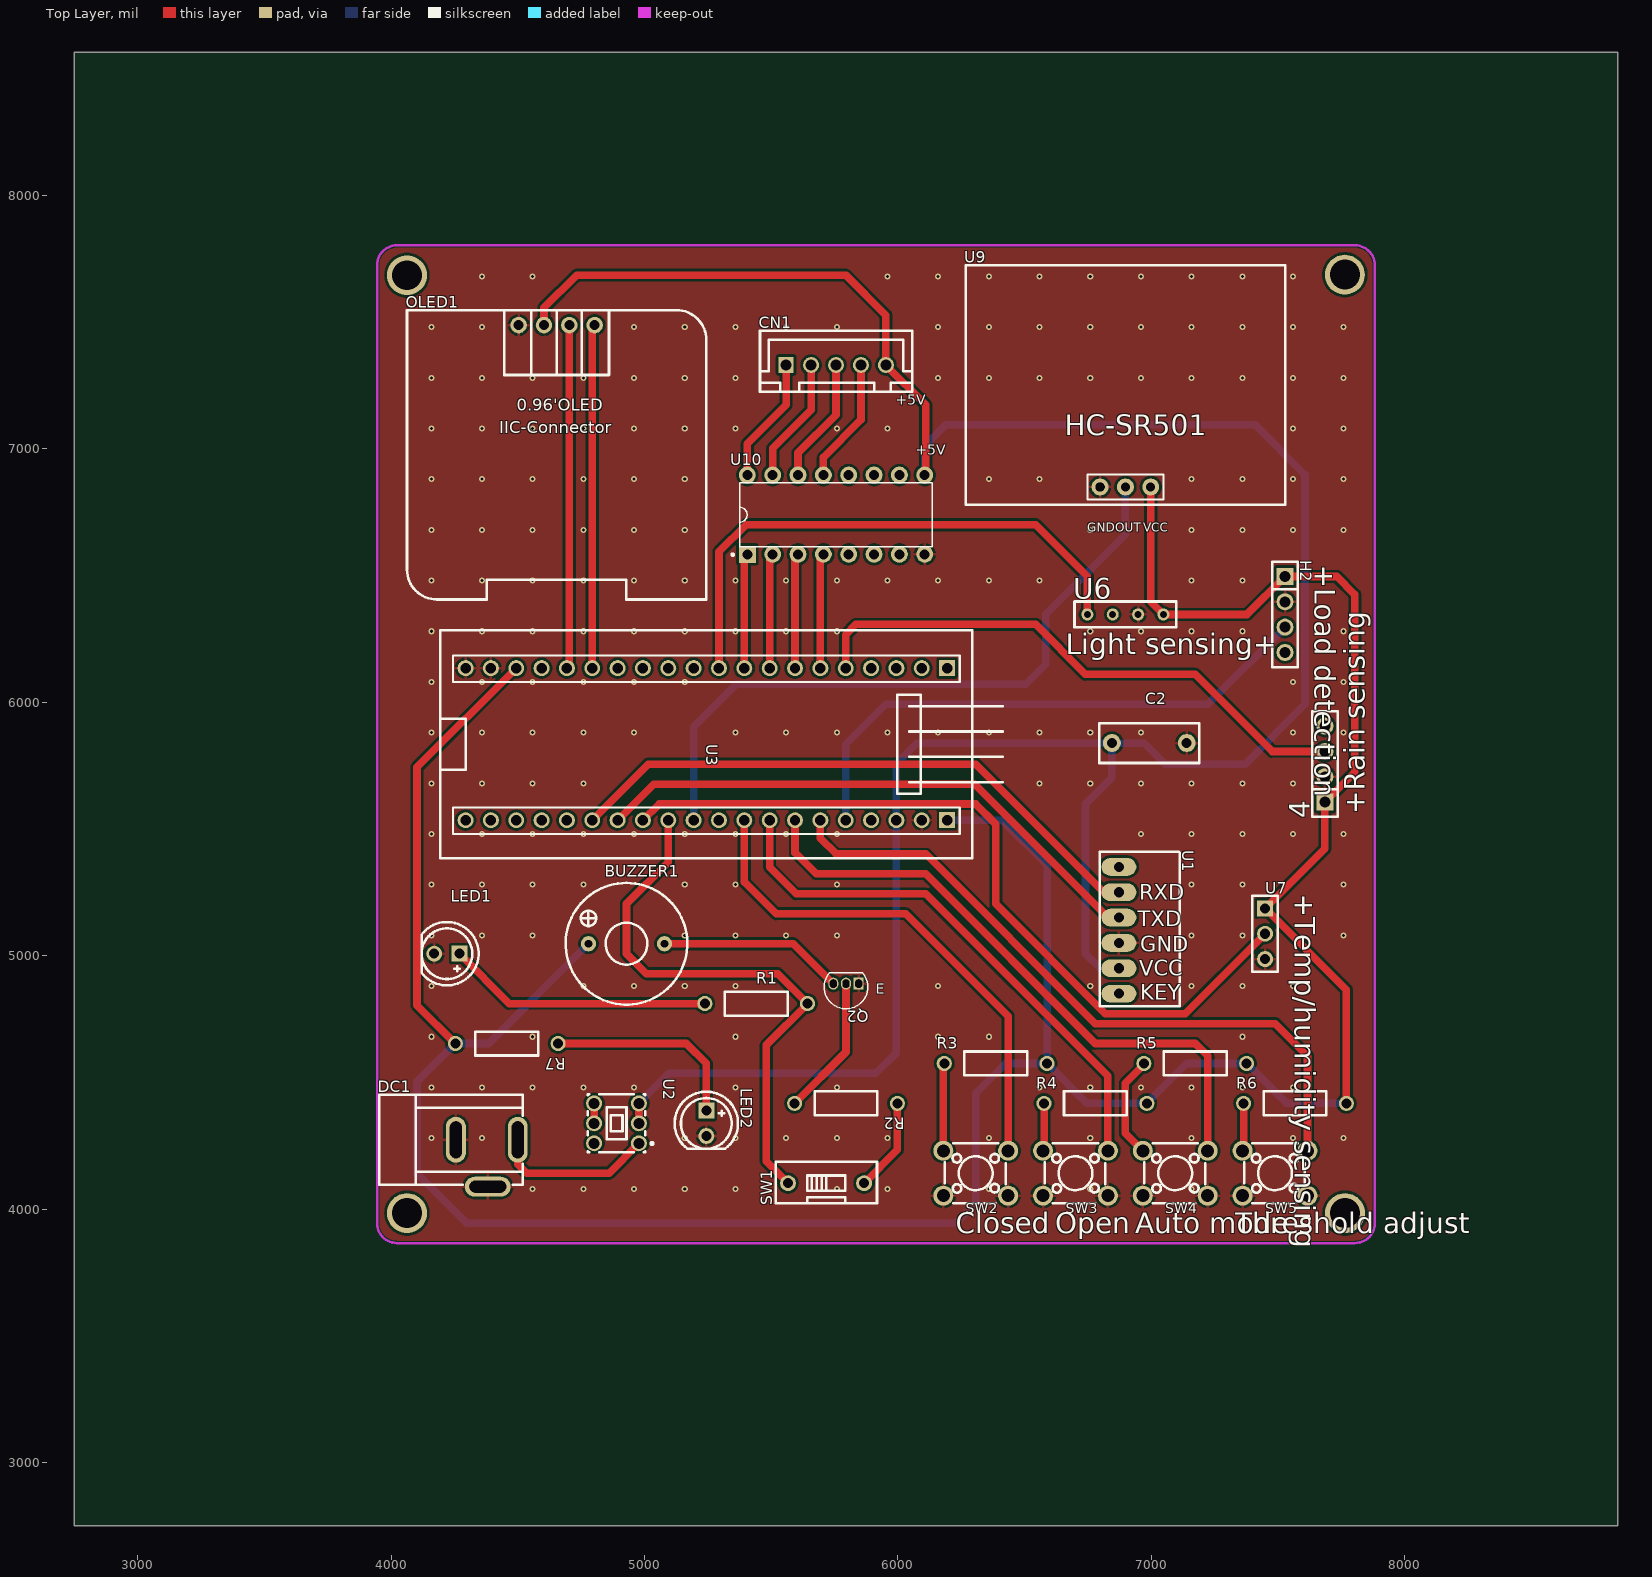
[diagram p0: Top Layer view]
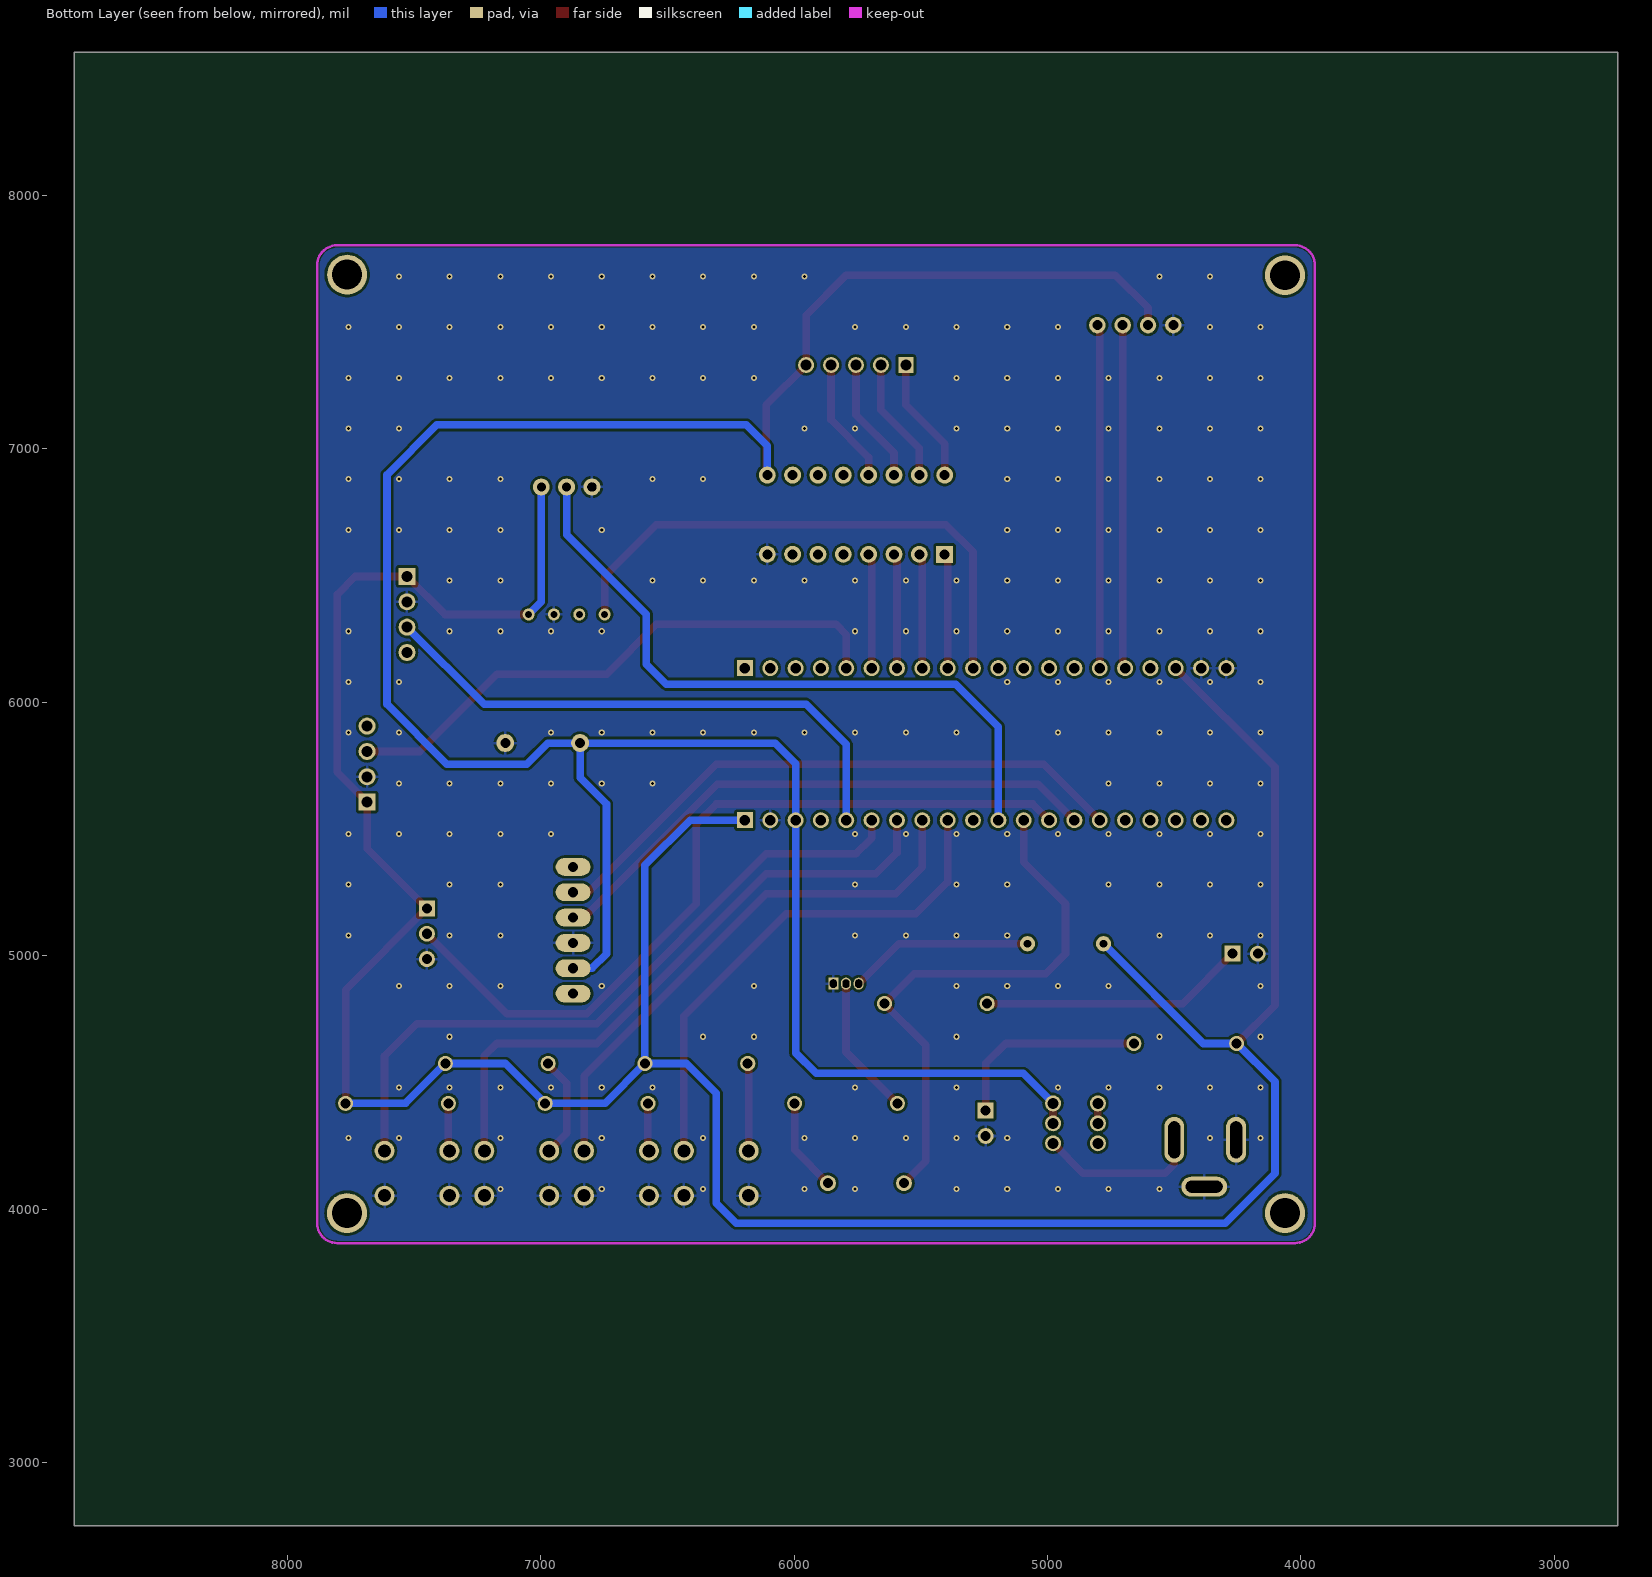
[diagram p1: Bottom Layer view, seen from below]
# Altium PCB MISC61241.pcbdoc
Units mil, origin at the board's own origin, x right, y up, seen from the top; angles counter-clockwise.
Board outline 6090.55 x 5814.96 mil, 2 copper layers (Top Layer, Bottom Layer), stack 62.206 mil thick; 29 components, 36 nets, 145 pads, 225 vias.

## Layer stack, top to bottom
Top Solder Mask Layer: solder mask 0.394, Dk 3.3
Top Layer: signal copper 1.379
Dielectric1: surface 59.449, FR4, Dk 4.5
Bottom Layer: signal copper 1.378
Bottom Solder Mask Layer: solder mask 0.394, Dk 3.3

## Board outline
8840.55,2750 2750,2750 2750,8564.96 8840.55,8564.96

## Design rules (kind name [scope] priority, off if disabled: settings)
BoardOutlineClearance copperThickness2oz_1 [All] p2 off: genericclearance=7.99 ignorepadtopadclearanceinfootprint=FALSE except(0: Arc-SplitContinuation Track-SplitContinuation SMDPad-SplitContinuation THPad-SplitContinuation Via-SplitContinuation Fill-SplitContinuation Region-SplitContinuation Poly-SplitContinuation Text-SplitContinuation Hole-SplitContinuation; 5.98: Arc-CutoutEdge SMDPad-CutoutEdge THPad-CutoutEdge Via-CutoutEdge Fill-CutoutEdge Region-CutoutEdge Text-CutoutEdge; 6.93: Hole-OutlineEdge Hole-CutoutEdge; 10: Poly-OutlineEdge Poly-CutoutEdge; 11.81: Arc-OutlineEdge Track-OutlineEdge SMDPad-OutlineEdge THPad-OutlineEdge Via-OutlineEdge Fill-OutlineEdge Region-OutlineEdge Text-OutlineEdge Track-CutoutEdge)
BoardOutlineClearance copperThickness1oz_1 [All] p4: genericclearance=4.02 ignorepadtopadclearanceinfootprint=FALSE except(0: Arc-SplitContinuation Track-SplitContinuation SMDPad-SplitContinuation THPad-SplitContinuation Via-SplitContinuation Fill-SplitContinuation Region-SplitContinuation Poly-SplitContinuation Text-SplitContinuation Hole-SplitContinuation; 6: SMDPad-CutoutEdge THPad-CutoutEdge Via-CutoutEdge Fill-CutoutEdge Region-CutoutEdge Text-CutoutEdge; 6.93: Hole-OutlineEdge Hole-CutoutEdge; 10: Poly-OutlineEdge Poly-CutoutEdge; 11.8: Arc-OutlineEdge Track-OutlineEdge SMDPad-OutlineEdge THPad-OutlineEdge Via-OutlineEdge Fill-OutlineEdge Region-OutlineEdge Text-OutlineEdge; 11.81: Arc-CutoutEdge Track-CutoutEdge)
Clearance copperThickness2oz [All] p1 off: gap=7.99 ignorepadtopadclearanceinfootprint=FALSE except(5.98: SMDPad-Track SMDPad-SMDPad THPad-Track SMDPad-THPad THPad-THPad Track-Via SMDPad-Via THPad-Via Via-Via Fill-Track Region-Track Fill-SMDPad Region-SMDPad Fill-THPad Region-THPad Fill-Via Region-Via Fill-Fill Fill-Region Region-Region Arc-Track Arc-SMDPad Arc-THPad Arc-Via Fill-Arc Region-Arc Arc-Arc Text-Track SMDPad-Text Text-THPad Text-Via Fill-Text Region-Text Arc-Text Text-Text; 6.93: Hole-Track Hole-SMDPad Hole-THPad Hole-Via Fill-Hole Region-Hole Hole-Arc Hole-Text; 10: Poly-Track Poly-SMDPad Poly-THPad Poly-Via Poly-Fill Poly-Region Poly-Poly Poly-Arc Poly-Text Poly-Hole)
Clearance copperThickness1oz [All] p3: gap=4.02 ignorepadtopadclearanceinfootprint=FALSE except(5.98: SMDPad-Track SMDPad-SMDPad THPad-Track SMDPad-THPad THPad-THPad Track-Via SMDPad-Via THPad-Via Via-Via Fill-Track Region-Track Fill-SMDPad Region-SMDPad Fill-THPad Region-THPad Fill-Via Region-Via Fill-Fill Fill-Region Region-Region; 6: Arc-Track Arc-SMDPad Arc-THPad Arc-Via Fill-Arc Region-Arc Arc-Arc Text-Track SMDPad-Text Text-THPad Text-Via Fill-Text Region-Text Arc-Text Text-Text; 6.93: Hole-Track Hole-SMDPad Hole-THPad Hole-Via Fill-Hole Region-Hole Hole-Arc Hole-Text; 10: Poly-Track Poly-SMDPad Poly-THPad Poly-Via Poly-Fill Poly-Region Poly-Poly Poly-Arc Poly-Text Poly-Hole)
DiffPairsRouting differentialPair [All] p1: maxlimit=6 minlimit=6 mostfreqgap=6 toplayer_minwidth=5 toplayer_prefwidth=10 toplayer_maxwidth=100 toplayer_mingap=6 toplayer_prefgap=6 toplayer_maxgap=6 bottomlayer_minwidth=5 bottomlayer_prefwidth=10 bottomlayer_maxwidth=100 bottomlayer_mingap=6 bottomlayer_prefgap=6 bottomlayer_maxgap=6 maxuncoupledlength=10
HoleToHoleClearance otherClearance [All] p1: gap=11.81 allowstackedmicrovias=TRUE
Length netLength [All] p1: minlimit=0 maxlimit=0
MatchedLengths netLengthTolerance [All] p1: tolerance=1000
PasteMaskExpansion pasteMaskExpansion [All] p1: expansion=0
PlaneConnect innerPlane [All] p1: planeconnectstyle=Relief reliefexpansion=20 reliefentries=4 reliefconductorwidth=10 reliefairgap=10
PolygonConnect "copperRegion_Top Layer" [(InNet('GND')) And OnLayer('Top Layer')] p1: connectstyle=Relief reliefconductorwidth=10 reliefentries=4 polygonreliefangle="90 Angle" airgapwidth=10 via.connectstyle=Relief via.reliefconductorwidth=10 via.reliefentries=4 via.polygonreliefangle="90 Angle" via.airgapwidth=10
PolygonConnect "copperRegion_Bottom Layer" [(InNet('GND')) And OnLayer('Bottom Layer')] p2: connectstyle=Relief reliefconductorwidth=10 reliefentries=4 polygonreliefangle="90 Angle" airgapwidth=10 via.connectstyle=Relief via.reliefconductorwidth=10 via.reliefentries=4 via.polygonreliefangle="90 Angle" via.airgapwidth=10
PolygonConnect copperRegion [(InNet('GND'))] p3: connectstyle=Direct reliefconductorwidth=10 reliefentries=4 polygonreliefangle="90 Angle" airgapwidth=10 via.connectstyle=Relief via.reliefconductorwidth=10 via.reliefentries=4 via.polygonreliefangle="90 Angle" via.airgapwidth=10
RoutingVias viaSize [All] p1: holewidth=12.01 width=24.02 viastyle="Through Hole" minholewidth=11.81 minwidth=19.68 maxholewidth=248.03 maxwidth=393.7
SolderMaskExpansion solderMaskExpansion [IsVia] p1: expansion=-1000 istentingtop=TRUE
SolderMaskExpansion solderMaskExpansion [All] p2: expansion=2 istentingtop=FALSE
Width copperThickness2oz_2 [All] p1 off: maxlimit=10 minlimit=10 preferedwidth=10 toplayer_minwidth=8 toplayer_maxwidth=100 toplayer_prefwidth=10 bottomlayer_minwidth=8 bottomlayer_maxwidth=100 bottomlayer_prefwidth=10
Width power [(InNet('+5V') OR InNet('GND') OR InNet('+3.3V') OR InNet('IN_5V'))] p2: maxlimit=10 minlimit=10 preferedwidth=10 toplayer_minwidth=10 toplayer_maxwidth=100 toplayer_prefwidth=20 bottomlayer_minwidth=10 bottomlayer_maxwidth=100 bottomlayer_prefwidth=20
Width copperThickness1oz_2 [All] p3: maxlimit=10 minlimit=10 preferedwidth=10 toplayer_minwidth=5 toplayer_maxwidth=100 toplayer_prefwidth=10 bottomlayer_minwidth=5 bottomlayer_maxwidth=100 bottomlayer_prefwidth=10

## Components (designator, comment, footprint, x,y, rotation, side; value= is the part's Value field where it differs from the comment)
4 "" HDR-TH_4P-P2.54-V-F 7685.04,5755.91 r90 top
BUZZER1 "3kHz" BUZZER 4929.13,5047.24 r90 top
C2 "10uF" CAP-TH_L10.0-W4.0-P7.50-D0.6-1 6992.1,5839.07 r180 top
CN1 "HX-XH2.54-5PZZ" CONN-TH_5P-P2.50_ZX-XH2.54-5PZZ 5755.91,7330.71 r0 top
DC1 "DC005" DC-IN-TH_DC005 4377.95,4181.1 r0 top
H2 "" HDR-TH_4P-P2.54-V-F 7527.56,6346.46 r270 top
LED1 "" LED-TH_5mm 4220.47,5007.87 r180 top
LED2 "" LED-TH_5mm 5244.09,4338.58 r270 top
OLED1 "" 0.96OLED_4P 4653.54,7488.19 r0 top
Q2 "S8050" TO-92-3_L4.5-W3.5-P1.27-L 5795.28,4889.76 r180 top
R1 "1K" Res_1/4W 5440.94,4811.02 r0 top
R2 "10kΩ" Res_1/4W 5795.28,4417.32 r180 top
R3 "10kΩ" Res_1/4W 6385.83,4574.8 r0 top
R4 "10kΩ" Res_1/4W 6779.53,4417.32 r0 top
R5 "10kΩ" Res_1/4W 7173.23,4574.8 r0 top
R6 "10kΩ" Res_1/4W 7566.93,4417.32 r0 top
R7 "1K" Res_1/4W 4456.69,4653.54 r180 top
SW1 "DIP switch" SW-TH_DSWB01LHGET 5716.54,4102.36 r90 top
SW2 "Tact switch" KEY-TH_4P-L6.0-W6.0-P4.50-LS6.50 6307.09,4141.73 r180 top
SW3 "Tact switch" KEY-TH_4P-L6.0-W6.0-P4.50-LS6.50 6700.79,4141.73 r180 top
SW4 "Tact switch" KEY-TH_4P-L6.0-W6.0-P4.50-LS6.50 7094.49,4141.73 r180 top
SW5 "Tact switch" KEY-TH_4P-L6.0-W6.0-P4.50-LS6.50 7488.19,4141.73 r180 top
U1 "HC05" HC05 5677.17,-14834.65 r270 top
U2 "Self-lock switch" SW-TH_6P-L5.8-W5.8-P2.00-LS4.5-TR 4889.76,4338.58 r270 top
U3 "STM32F103C8T6" STM32F103C8T6核心板 5244.09,5834.65 r270 top
U6 "" HDR-TH_4P-P2.54_342-40-104-00-592000 6897.64,6346.46 r0 top
U7 "" HDR-TH_3P-P2.54-V-M-B 7448.82,5086.61 r90 top
U9 "HC-SR501 human infrared sensor" 大闸蟹-HC-SR501人体红外传感器 6267.72,6779.53 r0 top
U10 "ULN2003AN(XBLW)" PDIP-16_L19.3-W6.4-P2.54-LS7.9-BL 5755.91,6740.16 r0 top

## Footprints (in the part's own frame and the unit in brackets; to place one, negate y for a bottom-side part, rotate by r counter-clockwise, add the part's x,y. Pads: shape width x height; smd on the part's side, far side on the other; paste and mask are expansions set on the pad)
0.96OLED_4P [mm]
  round 1.65 hole 1 copper offset 0,0: 1(-3.81,-0.001) 2(-1.27,0.002) 3(1.27,0.002) 4(3.81,0.002)
  silkscreen extent -15,-27.5 15,1.5
BUZZER [mil]
  round 60 hole 30: 1(0,150) 2(0,-150)
  silkscreen extent -240,-240 240,240
CAP-TH_L10.0-W4.0-P7.50-D0.6-1 [mm]
  round 1.8 hole 1: 1(-3.75,0) 2(3.75,0)
  silkscreen extent -5,-2 5,2
CONN-TH_5P-P2.50_ZX-XH2.54-5PZZ [mm]
  rect 1.524x1.6 hole 1.1: 1(-5,0)
  round 1.6 hole 1.1: 2(-2.5,0) 3(0,0) 4(2.5,0) 5(5,0)
  silkscreen extent -7.62,-2.68 7.62,3.42
DC-IN-TH_DC005 [mm]
  oval 2x4.6 hole 1.2 slot 3.7 at 90 deg: 1(3.1,2.35) 2(-3.1,2.35)
  oval 4.6x2 hole 1.2 slot 3.7 at 0 deg: 3(0.1,-2.35)
  silkscreen extent -10.8,-2.15 3.6,6.85
HC05 [mil]
  oval 70x137.8 hole 40 paste+0 mask+4: 1(-20185,1195) 2(-20085,1195) 3(-19985,1195) 4(-19885,1195) 5(-19785,1195) 6(-19685,1195)
  silkscreen extent -20245,1120 -19635,1435
HDR-TH_3P-P2.54-V-M-B [mm]
  rect 1.6x1.6 hole 1.02: 1(2.54,0)
  round 1.6 hole 1.02: 2(0,0) 3(-2.54,0)
  silkscreen extent -3.81,-1.27 3.81,1.27
HDR-TH_4P-P2.54-V-F [mm]
  rect 1.7x1.7 hole 1.1: 1(-3.81,0)
  round 1.7 hole 1.1: 2(-1.27,0) 3(1.27,0) 4(3.81,0)
  silkscreen extent -5.29,-1.27 5.29,1.27
HDR-TH_4P-P2.54_342-40-104-00-592000 [mm]
  round 1.2 hole 0.7: 1(-3.81,0) 2(-1.27,0) 3(1.27,0) 4(3.81,0)
  silkscreen extent -5.1,-1.3 5.1,1.3
KEY-TH_4P-L6.0-W6.0-P4.50-LS6.50 [mm]
  round 2 hole 1.3: 1(-3.25,2.25) 2(3.25,2.25) 3(-3.25,-2.25) 4(3.25,-2.25)
  silkscreen extent -3,-3 3.1,3
LED-TH_5mm [mm]
  rect 1.6x1.6 hole 1 paste+0 mask+0.051: 1(-1.27,0)
  round 1.6 hole 1 paste+0 mask+0.051: 2(1.27,0)
  silkscreen extent -3.17,-3.17 2.54,3.17
PDIP-16_L19.3-W6.4-P2.54-LS7.9-BL [mm]
  rect 1.7x1.7 hole 1: 1(-8.89,-3.97)
  round 1.7 hole 1 copper offset 0,0: 2(-6.35,-3.97) 3(-3.81,-3.97) 4(-1.27,-3.97) 5(1.27,-3.97) 6(3.81,-3.97) 7(6.35,-3.97) 8(8.89,-3.97)
  round 1.7 hole 1: 9(8.89,3.97) 10(6.35,3.97) 11(3.81,3.97) 12(1.27,3.97) 13(-1.27,3.97) 14(-3.81,3.97) 15(-6.35,3.97) 16(-8.89,3.97)
  silkscreen extent -10.46,-4.1 9.65,3.2
Res_1/4W [mil]
  round 60 hole 39.37 paste+0 mask+2: 1(-202.76,0) 2(202.76,0)
  silkscreen extent -124,-47 124,47
STM32F103C8T6核心板 [mil]
  rect 63x63 hole 41.3 paste+4 mask+4: 1(-300,950) 40(300,950)
  round 63 hole 41.3 paste+4 mask+4: 2(-300,850) 3(-300,750) 4(-300,650) 5(-300,550) 6(-300,450) 7(-300,350) 8(-300,250) 9(-300,150) 10(-300,50) 11(-300,-50) 12(-300,-150) 13(-300,-250) 14(-300,-350) 15(-300,-450) 16(-300,-550) 17(-300,-650) 18(-300,-750) 19(-300,-850) 20(-300,-950) 21(300,-950) 22(300,-850) 23(300,-750) 24(300,-650) 25(300,-550) 26(300,-450) 27(300,-350) 28(300,-250) 29(300,-150) 30(300,-50) 31(300,50) 32(300,150) 33(300,250) 34(300,350) 35(300,450) 36(300,550) 37(300,650) 38(300,750) 39(300,850)
  silkscreen extent -450,-1050 450,1169
SW-TH_6P-L5.8-W5.8-P2.00-LS4.5-TR [mm]
  round 1.6 hole 1.1: 1(2,2.25) 2(0,2.25) 3(-2,2.25) 4(-2,-2.25) 5(0,-2.25) 6(2,-2.25)
  silkscreen extent -2.9,-2.9 2.9,3.68
SW-TH_DSWB01LHGET [mm]
  round 1.6 hole 1: 1(0,3.81) 2(0,-3.81)
  silkscreen extent -2.02,-5.11 2.13,5.05
TO-92-3_L4.5-W3.5-P1.27-L [mm]
  rect 1x1.2 hole 0.7 slot 0.85 at 90 deg: 1(-1.27,0)
  oval 1x1.2 hole 0.7 slot 0.85 at 90 deg: 2(0,0) 3(1.27,0)
  silkscreen extent -2.19,-1.1 2.19,2.52
大闸蟹-HC-SR501人体红外传感器 [mil]
  round 66.93 hole 35.43 slot 35.63 at 0 deg paste+0 mask+4: 1(530,70)
  round 66.93 hole 35.43 paste+0 mask+4: 2(630,70) 3(730,70)
  silkscreen extent 0,0 1260,945

## Free pads (board coordinates)
  round 157.48 hole 118.11: 1(4062.99,3984.25) 1(4062.99,7685.04) 1(7763.78,7687.32) 1(7764.26,3984.25)

## Via types
v1: diameter 24.02, hole 12, Top Layer to Bottom Layer, 225 vias

## Nets (pads, with @x,y where several pads share a name; then routed paths per layer and width w, separated by ;. In a path a pad name is that pad's centre, name@x,y a point inside that pad or via, vN(x,y) a via of type N, cw(c..) or ccw(c..) an arc to the next point about the centre after c; other vN are vias at no path point)
$1N15: U2.4 U2.5 | length 78.7
  Top Layer w30: U2.5 U2.4
$1N17: BUZZER1.2 Q2.3 | length 731.4
  Top Layer w30: BUZZER1.2 5587.8,5047.24 Q2.3
$1N24: LED1.1 R1.1 | length 1049.3
  Top Layer w30: LED1.1 4467.32,4811.02 R1.1
$1N26: R2.1 SW1.2 | length 369.4
  Top Layer w30: SW1.2 5998.04,4233.86 R2.1
$1N40: R3.1 SW2.4 | length 346.1
  Top Layer w30: SW2.4 6179.14,4570.87 R3.1
$1N46: R4.1 SW3.4 | length 188.6
  Top Layer w30: SW3.4 6576.77,4234.24 R4.1
$1N50: R5.1 SW4.4 | length 403.2
  Top Layer w30: SW4.4 6897.64,4299.21 6897.64,4496.06 6970.47,4568.89 R5.1
$1N54: R6.1 SW5.4 | length 188.6
  Top Layer w30: SW5.4 7364.17,4234.24 R6.1
$1N67: LED2.1 R7.1 | length 803.5
  Top Layer w30: R7.1@4659.45,4653.54 5165.35,4653.54 5244.09,4574.8 LED2.1
$1N77: CN1.1 U10.16 | length 497.7
  Top Layer w30: U10.16 5405.91,7020.08 5559.05,7173.22 CN1.1
$1N78: CN1.2 U10.15 | length 497
  Top Layer w30: U10.15 5505.91,7001.97 5657.48,7153.54 CN1.2
$1N79: CN1.3 U10.14 | length 496.4
  Top Layer w30: U10.14 5605.91,6983.86 5755.9,7133.85 CN1.3
$1N80: CN1.4 U10.13 | length 495.7
  Top Layer w30: U10.13 5705.91,6965.75 5854.33,7114.17 CN1.4
$1N136: Q2.2 R2.2 | length 556.4
  Top Layer w30: R2.2 5795.28,4620.08 Q2.2
+3.3V: 4.1 BUZZER1.1 H2.1 R3.2 R4.2 R5.2 R6.2 R7.2 U3.18 U3.40 U6.4 U7.1 U9.3 | length 12860.3
  Top Layer w30: R7.2 4102.36,4805.11 4102.36,5742.91 U3.18 ; U9.3 6997.72,6396.38 U6.4 7377.56,6346.46 H2.1 7731.89,6496.46 7803.15,6425.2 7803.15,5724.02 4.1 7685.04,5422.83 U7.1 7769.69,4865.74 R6.2
  Bottom Layer w30: BUZZER1.1 4385.43,4653.54 R7.2 4102.36,4501.97 4102.36,4141.73 4299.21,3944.88 6228.35,3944.88 6307.09,4023.62 6307.09,4456.69 6425.2,4574.8 R3.2 ; U3.40 6410.24,5534.65 6588.59,5356.3 R3.2 ; U9.3 6997.72,6396.38 U6.4 ; R6.2 7533.47,4417.32 R5.2 7139.77,4574.8 R4.2 6746.07,4417.32 R3.2
+5V: C2.2 CN1.5 OLED1.2 U1.5 U2.2 U2.3 U3.38 U10.9 | length 9997.7
  Top Layer w30: OLED1.2@4603.54,7488.24 4603.54,7556.3 4732.28,7685.04 5795.28,7685.04 5952.76,7527.55 CN1.5 6110.24,7173.23 6110.24,6900.79 U10.9 ; U2.2 U2.3
  Bottom Layer w30: U2.3 5096.45,4535.43 5913.39,4535.43 5994.09,4616.14 U3.38 5994.09,5757.87 6075.3,5839.07 C2.2 ; U10.9 6105.91,7011.42 6188.98,7094.49 7409.45,7094.49 7606.3,6897.64 7606.3,5992.13 7370.08,5755.91 7055.12,5755.91 6971.95,5839.07 C2.2 ; U1.5 6797.68,4950.35 6740.16,5007.87 6740.16,5598.43 6844.46,5702.72 C2.2
GND: 4.2 C2.1 DC1.2 DC1.3 H2.2 LED1.2 LED2.2 OLED1.1 Q2.1 SW2.1 SW2.2 SW3.1 SW3.2 SW4.1 SW4.2 SW5.1 SW5.2 U1.4 U3.19 U3.20 U3.39 U6.3 U7.3 U9.1 U10.8
  other v1: 4558.98,4080.24 4758.98,4080.24 4958.98,4080.24 5158.98,4080.24 5358.98,4080.24 5758.98,4080.24 5958.98,4080.24 6358.98,4080.24 6758.98,4080.24 7158.98,4080.24 4158.98,4280.24 4358.98,4280.24 5158.98,4280.24 5358.98,4280.24 5558.98,4280.24 5758.98,4280.24 5958.98,4280.24 6358.98,4280.24 6758.98,4280.24 7158.98,4280.24 7558.98,4280.24 7758.98,4280.24 4158.98,4480.24 4358.98,4480.24 4558.98,4480.24 4758.98,4480.24 4958.98,4480.24 5358.98,4480.24 5758.98,4480.24 6558.98,4480.24 6758.98,4480.24 6958.98,4480.24 7158.98,4480.24 7358.98,4480.24 7558.98,4480.24 4158.98,4680.24 4558.98,4680.24 5358.98,4680.24 6158.98,4680.24 6358.98,4680.24 7358.98,4680.24 4158.98,4880.24 4758.98,4880.24 4958.98,4880.24 5158.98,4880.24 5358.98,4880.24 6158.98,4880.24 6758.98,4880.24 7158.98,4880.24 7358.98,4880.24 7558.98,4880.24 4158.98,5080.24 4358.98,5080.24 4558.98,5080.24 5158.98,5080.24 5358.98,5080.24 5558.98,5080.24 5758.98,5080.24 7158.98,5080.24 7358.98,5080.24 7758.98,5080.24 4158.98,5280.24 4358.98,5280.24 4558.98,5280.24 4758.98,5280.24 5158.98,5280.24 5358.98,5280.24 5758.98,5280.24 7158.98,5280.24 7358.98,5280.24 7758.98,5280.24 4158.98,5480.24 4358.98,5480.24 4558.98,5480.24 4758.98,5480.24 4958.98,5480.24 5158.98,5480.24 5358.98,5480.24 5558.98,5480.24 5758.98,5480.24 6958.98,5480.24 7158.98,5480.24 7358.98,5480.24 7558.98,5480.24 7758.98,5480.24 4158.98,5680.24 4358.98,5680.24 4558.98,5680.24 4758.98,5680.24 6558.98,5680.24 6758.98,5680.24 6958.98,5680.24 7158.98,5680.24 7358.98,5680.24 7558.98,5680.24 4158.98,5880.24 4358.98,5880.24 4558.98,5880.24 4758.98,5880.24 4958.98,5880.24 5358.98,5880.24 5558.98,5880.24 5758.98,5880.24 5958.98,5880.24 6158.98,5880.24 6358.98,5880.24 6558.98,5880.24 6758.98,5880.24 6958.98,5880.24 7558.98,5880.24 7758.98,5880.24 4158.98,6080.24 4358.98,6080.24 4558.98,6080.24 4758.98,6080.24 4958.98,6080.24 5158.98,6080.24 7558.98,6080.24 7758.98,6080.24 4158.98,6280.24 4358.98,6280.24 4558.98,6280.24 4758.98,6280.24 4958.98,6280.24 5158.98,6280.24 5358.98,6280.24 5558.98,6280.24 5758.98,6280.24 6758.98,6280.24 6958.98,6280.24 7158.98,6280.24 7358.98,6280.24 7758.98,6280.24 4158.98,6480.24 4358.98,6480.24 4558.98,6480.24 4758.98,6480.24 4958.98,6480.24 5158.98,6480.24 5358.98,6480.24 5558.98,6480.24 5758.98,6480.24 5958.98,6480.24 6158.98,6480.24 6358.98,6480.24 6558.98,6480.24 7158.98,6480.24 7358.98,6480.24 4158.98,6680.24 4358.98,6680.24 4558.98,6680.24 4758.98,6680.24 4958.98,6680.24 5158.98,6680.24 6758.98,6680.24 7158.98,6680.24 7358.98,6680.24 7558.98,6680.24 7758.98,6680.24 4158.98,6880.24 4358.98,6880.24 4558.98,6880.24 4758.98,6880.24 4958.98,6880.24 5158.98,6880.24 6358.98,6880.24 6558.98,6880.24 7158.98,6880.24 7358.98,6880.24 7558.98,6880.24 7758.98,6880.24 4158.98,7080.24 4358.98,7080.24 4558.98,7080.24 4758.98,7080.24 4958.98,7080.24 5158.98,7080.24 5358.98,7080.24 5758.98,7080.24 5958.98,7080.24 7558.98,7080.24 7758.98,7080.24 4158.98,7280.24 4358.98,7280.24 4558.98,7280.24 4758.98,7280.24 4958.98,7280.24 5158.98,7280.24 5358.98,7280.24 6158.98,7280.24 6358.98,7280.24 6558.98,7280.24 6758.98,7280.24 6958.98,7280.24 7158.98,7280.24 7358.98,7280.24 7558.98,7280.24 7758.98,7280.24 4158.98,7480.24 4358.98,7480.24 4958.98,7480.24 5158.98,7480.24 5358.98,7480.24 5558.98,7480.24 5758.98,7480.24 6158.98,7480.24 6358.98,7480.24 6558.98,7480.24 6758.98,7480.24 6958.98,7480.24 7158.98,7480.24 7358.98,7480.24 7558.98,7480.24 7758.98,7480.24 4358.98,7680.24 4558.98,7680.24 5958.98,7680.24 6158.98,7680.24 6358.98,7680.24 6558.98,7680.24 6758.98,7680.24 6958.98,7680.24 7158.98,7680.24 7358.98,7680.24 7558.98,7680.24
IN_5V: DC1.1 U2.1 | length 638.4
  Top Layer w30: DC1.1 4499.99,4177.17 4535.43,4141.73 4860.23,4141.73 U2.1
PA0: 4.3 U3.5 | length 2247.2
  Top Layer w30: U3.5 5794.09,6266.54 5834.65,6307.09 6543.31,6307.09 6740.16,6110.24 7173.23,6110.24 7477.56,5805.91 4.3
PA1: U3.6 U10.4 | length 454.1
  Top Layer w30: U3.6 5694.09,6572.05 U10.4@5705.91,6583.86
PA2: U3.7 U10.3 | length 454.1
  Top Layer w30: U3.7 5594.09,6572.05 U10.3@5605.91,6583.86
PA3: U3.8 U10.2 | length 454.1
  Top Layer w30: U3.8 5494.09,6572.05 U10.2@5505.91,6583.86
PA4: U3.9 U10.1 | length 454.1
  Top Layer w30: U3.9 5394.09,6572.05 U10.1
PA5: U3.10 U6.1 | length 2191.4
  Top Layer w30: U3.10 5294.09,6593.31 5401.57,6700.79 6543.31,6700.79 6747.64,6496.46 U6.1
PA9: U1.2 U3.26 | length 2379.1
  Top Layer w30: U3.26 5015.35,5755.91 6307.09,5755.91 6812.64,5250.35 U1.2
PA10: U1.3 U3.27 | length 2255.3
  Top Layer w30: U3.27 5036.61,5677.17 6302.93,5677.17 6829.74,5150.35 U1.3
PA11: U3.28 U7.2 | length 3138.6
  Top Layer w30: U3.28 5057.87,5598.43 6307.09,5598.43 6385.83,5519.69 6385.83,5204.72 6818.9,4771.65 7133.86,4771.65 U7.2
PA12: R1.2 SW1.1 U3.29 | length 2203.3
  Top Layer w30: U3.29 5094.09,5369.69 4929.13,5204.72 4929.13,5007.87 5007.87,4929.13 5525.59,4929.13 R1.2 5480.31,4647.63 5480.31,4188.58 SW1.1
PA15: U3.30 U9.2 | length 2689.4
  Bottom Layer w30: U3.30 5194.09,5902.76 5362.2,6070.87 6503.94,6070.87 6582.68,6149.61 6582.68,6346.46 6897.72,6661.5 U9.2
PB4: SW2.3 U3.32 | length 2035.3
  Top Layer w30: U3.32 5394.09,5290.94 5519.69,5165.35 6031.5,5165.35 6435.04,4761.81 SW2.3
PB5: SW3.3 U3.33 | length 2157
  Top Layer w30: U3.33 5494.09,5348.43 5598.43,5244.09 6110.24,5244.09 6828.74,4525.59 SW3.3
PB6: SW4.3 U3.34 | length 2463.1
  Top Layer w30: U3.34 5594.09,5405.91 5677.17,5322.83 6110.24,5322.83 6779.53,4653.54 7173.23,4653.54 7222.44,4604.33 SW4.3
PB7: SW5.3 U3.35 | length 2723.2
  Top Layer w30: U3.35 5694.09,5463.39 5755.91,5401.57 6110.24,5401.57 6779.53,4732.28 7488.19,4732.28 7616.14,4604.33 SW5.3
PB8: H2.3 U3.36 | length 2224.1
  Bottom Layer w30: U3.36 5794.09,5833.46 5952.76,5992.13 7223.23,5992.13 H2.3
PB10: OLED1.4 U3.15 | length 1357.5
  Top Layer w30: U3.15 4794.09,7478.79 OLED1.4@4803.54,7488.24
PB11: OLED1.3 U3.16 | length 1357.5
  Top Layer w30: U3.16 4703.54,6144.09 OLED1.3@4703.54,7488.24
pads on no net: 4.4 H2.4 U1.1 U1.6 U2.6 U3.1 U3.2 U3.3 U3.4 U3.11 U3.12 U3.13 U3.14 U3.17 U3.21 U3.22 U3.23 U3.24 U3.25 U3.31 U3.37 U6.2 U10.5 U10.6 U10.7 U10.10 U10.11 U10.12

## Polygon pours and split planes (outlines as drawn)
GND on Bottom Layer (solid, remove dead copper, pour order 2): 3000,8314.96 3000,3000 8590.55,3000 8590.55,8314.96
GND on Top Layer (solid, remove dead copper, pour order 0): 3590.55,8118.11 3590.55,3236.22 8275.59,3236.22 8275.59,8118.11

## Keep-outs
Board Outline Layer:
  lines w10: 3944.88,3944.88 3944.88,7724.41 cw(c4023.62,7724.41) 4023.62,7803.15 7803.15,7803.15 cw(c7803.15,7724.41) 7881.89,7724.41 7881.89,3944.88 cw(c7803.15,3944.88) 7803.15,3866.14 4023.62,3866.14 cw(c4023.62,3944.88) 3944.88,3944.88

## Silkscreen, mask and mechanical layers (free items; w line width, h text height)
Top Silkscreen Layer:
  text "+5V" at 5992.13,7173.23 h40
  text "+5V" at 6070.87,6976.38 h40
  text "+Load detection" at 7645.67,6543.31 h80 r270
  text "Light sensing+" at 6661.42,6188.98 h80
  text "+Rain sensing" at 7842.52,5559.06 h80 r90
  text "+Temp/humidity sensing" at 7566.93,5244.09 h80 r270
  text "E" at 5913.39,4850.39 h40
  text "Closed" at 6228.35,3905.51 h80
  text "Auto mode" at 6937.01,3905.51 h80
  text "Threshold adjust" at 7330.71,3905.51 h80
  text "Open" at 6620.06,3904.88 h80